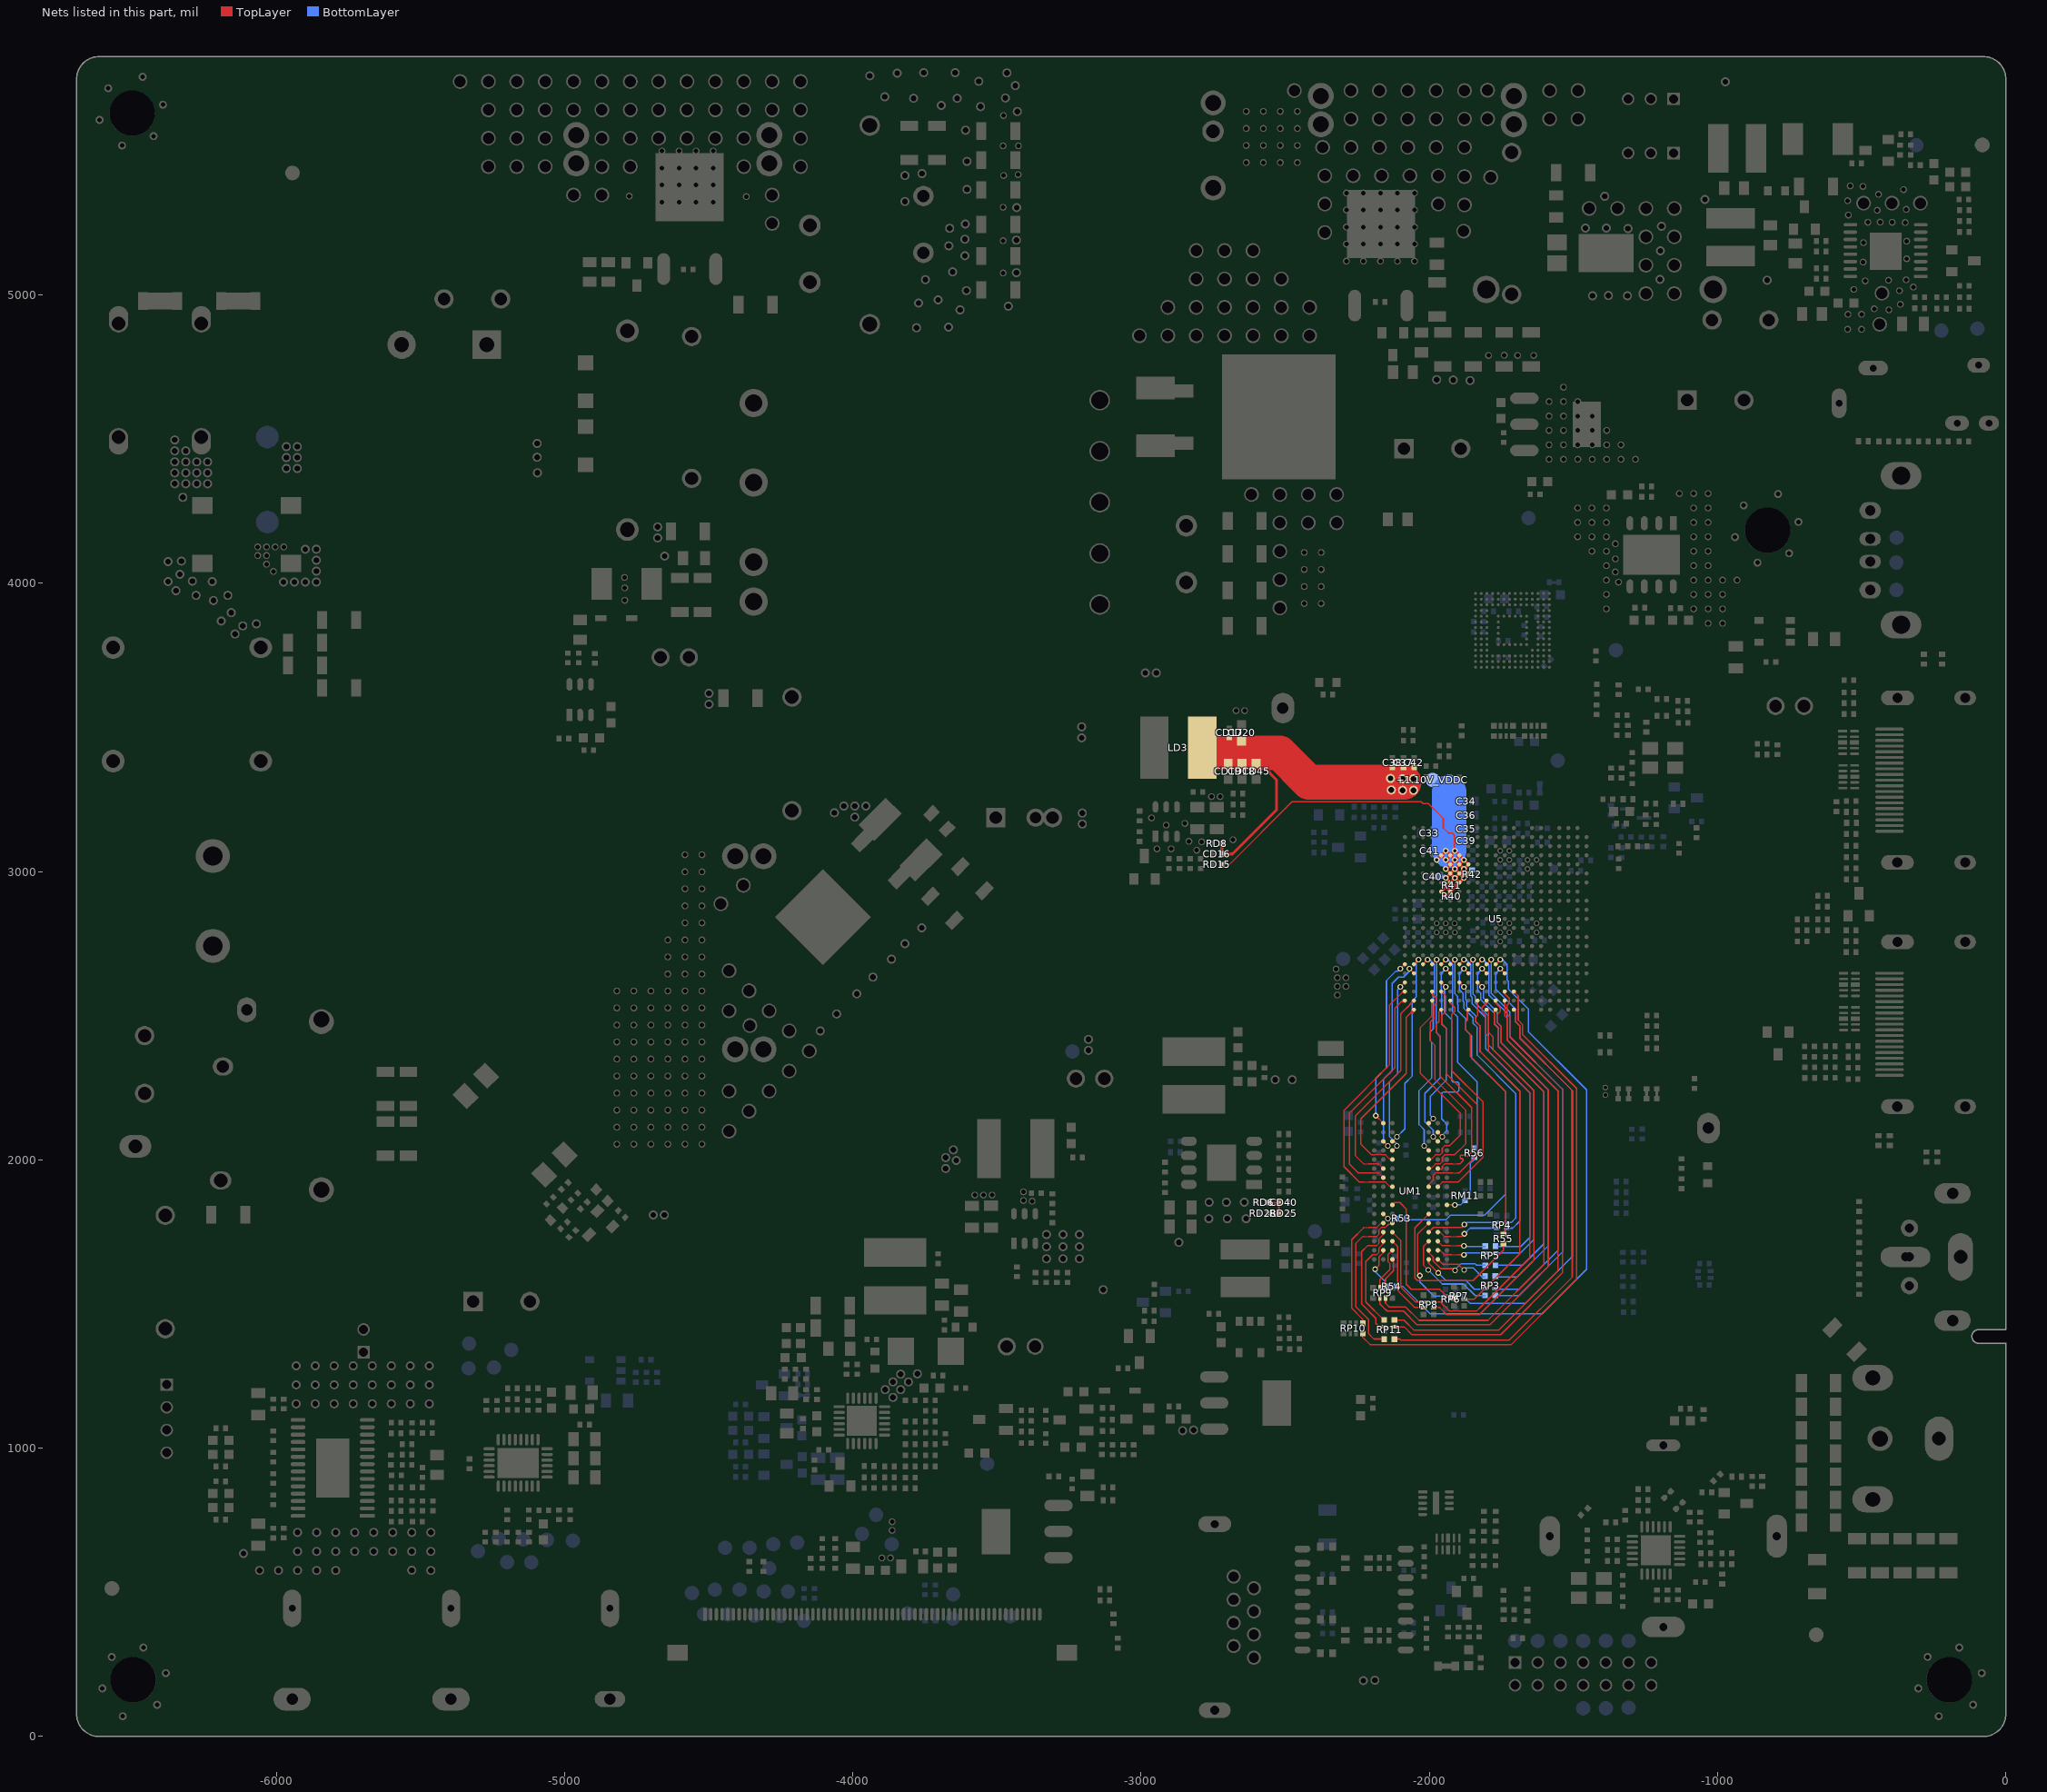
[diagram p0: the nets of this part, all layers, seen from the top]
# Altium PCB MISC84395.PcbDoc (part 10 of 26)
Units mil, origin at the board's own origin, x right, y up, seen from the top; angles counter-clockwise.
Board outline 6692.91 x 5826.77 mil, 2 copper layers (TopLayer, BottomLayer), stack 61.855 mil thick; 951 components, 565 nets, 4374 pads, 1804 vias.
Unrouted connection lines stored in the file: 1.

## Via types
v1: diameter 19.68, hole 11.81, TopLayer to BottomLayer, tented both sides, 1262 vias
v2: diameter 23.62, hole 15.75, TopLayer to BottomLayer, tented both sides, 524 vias
v3: diameter 31.5, hole 19.68, TopLayer to BottomLayer, tented both sides, 11 vias
v4: diameter 24, hole 16, TopLayer to BottomLayer, tented both sides, 6 vias
v5: diameter 19, hole 11.81, TopLayer to BottomLayer, tented both sides, 1 vias

## Nets (pads, with @x,y where several pads share a name; then routed paths per layer and width w, separated by ;. In a path a pad name is that pad's centre, name@x,y a point inside that pad or via, vN(x,y) a via of type N, cw(c..) or ccw(c..) an arc to the next point about the centre after c; other vN are vias at no path point) (continued)
+1.10V_VDDC: +1.10V_VDDC.1 C33.2 C34.2 C35.2 C36.2 C37.2 C38.2 C39.2 C40.2 C41.2 C42.2 CD16.2 CD17.1 CD18.1 CD19.1 CD20.1 CD45.1 LD3.2 pad.VIA5@-1880.2,2977.82 pad.VIA5@-1880.2,3009.31 pad.VIA5@-1880.2,3040.81 pad.VIA5@-1911.7,2977.82 pad.VIA5@-1911.7,3009.31 pad.VIA5@-1911.7,3040.81 pad.VIA5@-1911.7,3072.3 pad.VIA5@-1943.2,2977.82 pad.VIA5@-1943.2,3009.31 pad.VIA5@-1943.2,3040.81 pad.VIA5@-1943.2,3072.3 pad.VIA5@-1974.69,3040.81 pad.VIA5@-2055,3282 pad.VIA5@-2055,3322 pad.VIA5@-2093,3282 pad.VIA5@-2093,3322 pad.VIA5@-2132,3283 pad.VIA5@-2135,3323 R40.1 R41.1 R42.1 RD8.2 RD15.1 U5.P16 U5.P17 U5.R15 U5.R16 U5.T14 U5.T15 U5.T16 U5.U14 U5.U15 U5.U16 U5.V15 U5.V16 U5.V17 | length 3367.3
  TopLayer w5: RD15.1@-2720.27,3025.92 RD15.1@-2720.27,3024.19 -2694.01,3024.19 -2476.38,3241.82 -2028.06,3241.82 -2021.58,3235.34 -2002.82,3235.34 -1951.87,3184.4 -1951.87,3151.49 -1934.52,3134.14 -1921.41,3134.14 -1912.86,3125.59 -1912.86,3073.47 pad.VIA5@-1911.7,3072.3
  TopLayer w10: RD8.2@-2720.18,3097.93 CD16.2@-2720.18,3060.93 -2683.07,3060.93 -2530,3214 -2530,3318 -2575,3363 ; pad.VIA5@-1973.76,3041.74 U5.V17@-1958.94,3056.56 ; -1940.1,2943.22 U5.P16@-1927.45,2930.57 ; -1914.8,2949.42 U5.R16@-1927.45,2962.07 ; U5.V17@-1958.94,3056.56 pad.VIA5@-1943.2,3040.81 ; U5.V17@-1958.94,3056.56 pad.VIA5@-1943.2,3072.3 U5.V16@-1927.45,3056.56 ; pad.VIA5@-1943.2,3040.81 U5.V16@-1927.45,3056.56 ; pad.VIA5@-1943.2,3040.81 U5.U16@-1927.45,3025.06 ; U5.P16@-1927.45,2930.57 -1940.1,2917.92 -1946.3,2917.92 U5.P17@-1958.94,2930.57 U5.R16@-1927.45,2962.07 ; U5.P16@-1927.45,2930.57 -1908.6,2949.42 U5.R15@-1895.95,2962.07 ; U5.R16@-1927.45,2962.07 pad.VIA5@-1911.7,2977.82 ; U5.R16@-1927.45,2962.07 pad.VIA5@-1943.2,2977.82 U5.T16@-1927.45,2993.56 ; U5.T16@-1927.45,2993.56 pad.VIA5@-1911.7,3009.31 ; U5.T16@-1927.45,2993.56 pad.VIA5@-1911.7,2977.82 ; U5.T16@-1927.45,2993.56 pad.VIA5@-1943.2,3009.31 U5.U16@-1927.45,3025.06 ; U5.U16@-1927.45,3025.06 pad.VIA5@-1911.7,3040.81 ; U5.U16@-1927.45,3025.06 pad.VIA5@-1911.7,3009.31 ; U5.V16@-1927.45,3056.56 pad.VIA5@-1911.7,3040.81 ; U5.V16@-1927.45,3056.56 pad.VIA5@-1911.7,3072.3 U5.V15@-1895.95,3056.56 ; pad.VIA5@-1911.7,2977.82 U5.T15@-1895.95,2993.56 ; pad.VIA5@-1911.7,2977.82 U5.R15@-1895.95,2962.07 ; pad.VIA5@-1911.7,3009.31 U5.U15@-1895.95,3025.06 ; pad.VIA5@-1911.7,3009.31 U5.T15@-1895.95,2993.56 ; pad.VIA5@-1911.7,3040.81 U5.U15@-1895.95,3025.06 ; pad.VIA5@-1911.7,3040.81 U5.V15@-1895.95,3056.56 ; U5.R15@-1895.95,2962.07 pad.VIA5@-1880.2,2977.82 ; U5.T15@-1895.95,2993.56 pad.VIA5@-1880.2,2977.82 ; U5.T15@-1895.95,2993.56 pad.VIA5@-1880.2,3009.31 ; U5.U15@-1895.95,3025.06 pad.VIA5@-1880.2,3040.81 ; U5.U15@-1895.95,3025.06 pad.VIA5@-1880.2,3009.31 ; U5.V15@-1895.95,3056.56 pad.VIA5@-1880.2,3040.81 ; pad.VIA5@-1880.2,2977.82 U5.T14@-1864.46,2993.56 pad.VIA5@-1880.2,3009.31 ; pad.VIA5@-1880.2,3009.31 U5.U14@-1864.46,3025.06 pad.VIA5@-1880.2,3040.81
  TopLayer w120: LD3.2@-2774,3411.19 -2519.19,3411.19 -2418,3310 pad.VIA5@-2087,3310
  BottomLayer w12: -1931.35,3072.32 -1925.03,3066
  BottomLayer w15: C40.2@-1972.27,2982 pad.VIA5@-1947.38,2982
  BottomLayer w120: -1931.35,3072.32 -1931.35,3144.15 ; -1931.35,3146.15 -1931.35,3244.15 ; -1931.35,3242.15 -1931.35,3244.15 ; -1931.35,3275.47 -1931.35,3244.15
A2_EN: CD40.1 RD6.1 RD25.1 RD28.1 | length 160.9
  TopLayer w6: RD28.1@-2559.27,1814 RD25.1@-2521.73,1814 ; RD6.1@-2559.27,1851.73 RD6.1@-2559,1852 -2514.84,1852 -2521.73,1845.11 RD25.1@-2521.73,1814 ; CD40.1@-2521.73,1852 RD25.1@-2521.73,1814
A_DDR3_A0: RP8.3 UM1.N3 | length 302.9
  TopLayer w4.92: UM1.N3@-2128.24,1749.47 -2099.69,1720.92 -2099.69,1559.01 -2048.02,1507.34 RP8.3@-2020.46,1507.34
A_DDR3_A0_IC: RP8.4 U5.B12 | length 1382
  TopLayer w3.94: -1816.72,2513.74 -1817.21,2514.23 -1817.21,2528.99 -1801.47,2544.74 U5.B12@-1801.46,2552.62
  TopLayer w4.92: RP8.4@-1977.15,1507.34 -1961.9,1507.34 -1932.37,1477.82 -1930.81,1476.26 -1835.5,1476.26 -1821.52,1490.24 -1651.86,1659.9 -1651.86,2233.23 -1794.58,2375.94 -1794.58,2427.62 -1804.42,2437.46 -1804.42,2501.43 -1816.72,2513.74
A_DDR3_A1: RP3.1 UM1.P7 | length 349
  TopLayer w4.92: v1(-2003.73,1618.07) -2020.95,1635.29 -2020.95,1699.27 UM1.P7@-2002.25,1717.97
  BottomLayer w4.92: v1(-2003.73,1618.07) -1955.15,1569.49 -1881.34,1569.49 -1840.84,1529 RP3.1@-1806.38,1529
A_DDR3_A1_IC: RP3.2 U5.F12 | length 1426.2
  TopLayer w4.92: U5.F12@-1801.46,2678.6 v1(-1785.72,2694.35)
  BottomLayer w3.94: v1(-1785.72,2694.35) -1785.72,2578.7 -1785.23,2578.21
  BottomLayer w4.92: -1785.23,2578.21 -1720.76,2513.74 -1720.76,2427.62 -1538.67,2245.53 -1538.67,1679.59 -1689.26,1529 RP3.2@-1763.08,1529
A_DDR3_A2: RP8.5 UM1.P3 | length 292.5
  TopLayer w4.92: UM1.P3@-2128.24,1717.97 -2109.54,1699.27 -2109.54,1546.72 -2050.48,1487.66 RP8.5@-2020.46,1487.66
A_DDR3_A2_IC: RP8.6 U5.A12 | length 1365.4
  TopLayer w4.92: RP8.6@-1977.15,1487.66 -1964.36,1487.66 -1939.75,1463.05 -1826.55,1463.05 -1637.1,1652.52 -1637.1,2240.61 -1779.81,2383.32 -1779.81,2427.62 -1794.58,2442.38 -1794.58,2514.23 U5.A12@-1801.46,2521.12
A_DDR3_A3: RP11.3 UM1.N2 | length 418.6
  TopLayer w4.92: UM1.N2@-2159.73,1749.47 -2159.73,1741.59 -2175.48,1725.84 -2175.48,1710.1 -2183.36,1702.22 -2214.85,1702.22 -2235.03,1682.04 -2235.03,1499.96 -2185.81,1450.75 -2185.81,1433.52 -2173.51,1421.22 RP11.3@-2158.25,1421.22
A_DDR3_A3_IC: RP11.4 U5.C10 | length 1741.3
  TopLayer w3.94: U5.C10@-1738.47,2584.12 -1738.47,2576.24 -1722.73,2560.49 -1722.73,2544.74 -1730.6,2536.87 -1730.6,2506.36 -1730.11,2505.86
  TopLayer w4.92: RP11.4@-2114.95,1421.22 -2087.39,1421.22 -2060.32,1394.15 -1752.74,1394.15 -1538.67,1608.23 -1538.67,2245.53 -1720.76,2427.62 -1720.76,2496.51 -1730.11,2505.86
A_DDR3_A4: RP5.7 UM1.P8 | length 171.9
  TopLayer w3.94: -1927.45,1702.22 -1903.83,1702.23
  TopLayer w4.92: UM1.P8@-1970.75,1717.97 -1955.01,1702.22 -1927.45,1702.22 ; -1903.83,1702.23 v1(-1880.2,1702.23)
  BottomLayer w4.92: v1(-1880.2,1702.23) -1877.74,1699.77 RP5.7@-1806.38,1699.77
A_DDR3_A4_IC: RP5.8 U5.F15 | length 1208.8
  TopLayer w4.92: U5.F15@-1895.95,2678.6 v1(-1880.21,2694.35)
  BottomLayer w3.94: v1(-1880.21,2694.35) -1872.33,2694.35 -1856.58,2678.6 -1856.58,2568.36 -1856.09,2567.87
  BottomLayer w4.92: -1856.09,2567.87 -1851.17,2562.95 -1851.17,2540.8 -1804.42,2494.05 -1804.42,2385.78 -1651.86,2233.23 -1651.86,1731.26 -1683.35,1699.77 RP5.8@-1763.08,1699.77
A_DDR3_A5: RP11.1 UM1.P2 | length 332.9
  TopLayer w4.92: UM1.P2@-2159.73,1717.97 -2159.73,1710.1 -2175.48,1694.35 -2175.48,1678.6 -2183.36,1670.73 -2197.14,1670.73 -2220.26,1647.61 -2220.26,1507.34 -2158.25,1445.34 RP11.1@-2158.25,1443.86
A_DDR3_A5_IC: RP11.2 U5.B10 | length 1675.3
  TopLayer w3.94: U5.B10@-1738.47,2552.62 -1738.47,2499.47 -1737.98,2498.97
  TopLayer w4.92: RP11.2@-2114.95,1443.86 -2087.88,1443.86 -2052.94,1408.92 -1760.12,1408.92 -1553.43,1615.62 -1553.43,2238.15 -1730.6,2415.31 -1730.6,2491.59 -1737.98,2498.97
A_DDR3_A6: RP5.5 UM1.R8 | length 173.5
  TopLayer w3.94: -1923.51,1670.73 -1899.89,1670.73
  TopLayer w4.92: UM1.R8@-1970.75,1686.48 -1962.88,1686.47 -1947.14,1670.73 -1923.51,1670.73 ; -1899.89,1670.73 v1(-1880.2,1670.73)
  BottomLayer w4.92: v1(-1880.2,1670.73) -1873.81,1677.13 RP5.5@-1806.38,1677.13
A_DDR3_A6_IC: RP5.6 U5.F14 | length 1225.7
  TopLayer w4.92: U5.F14@-1864.46,2678.6 v1(-1848.71,2694.35)
  BottomLayer w3.94: v1(-1848.71,2694.35) -1848.71,2575.25 -1848.22,2574.76
  BottomLayer w4.92: -1848.22,2574.76 -1841.33,2567.87 -1841.33,2545.73 -1794.58,2498.97 -1794.58,2398.09 -1637.1,2240.61 -1637.1,1723.88 -1683.85,1677.13 RP5.6@-1763.08,1677.13
A_DDR3_A7: R54.1 UM1.R2 | length 151
  TopLayer w4.92: v1(-2188.27,1620.53) -2175.48,1633.33 -2175.48,1662.85 -2159.73,1678.6 UM1.R2@-2159.73,1686.48
  BottomLayer w4.92: v1(-2188.27,1620.53) -2188.27,1613.15 -2154.14,1579.02 R54.1@-2154.14,1561.48
A_DDR3_A7_IC: R54.2 U5.F11 | length 1987
  TopLayer w4.92: U5.F11@-1769.97,2678.6 v1(-1754.22,2694.35)
  BottomLayer w3.94: v1(-1754.22,2694.35) -1746.35,2694.35 -1730.6,2678.6 -1730.6,2624.47 -1730.11,2623.97
  BottomLayer w4.92: R54.2@-2114.14,1561.48 -2092.31,1561.48 -1998.81,1467.97 -1997.25,1466.42 -1609.12,1466.42 -1590.31,1485.23 -1455.01,1620.53 -1455.01,2243.07 -1656.78,2444.84 -1656.78,2523.58 -1725.68,2592.48 -1725.68,2619.54 -1730.11,2623.97
A_DDR3_A8: RP3.7 UM1.T8 | length 195.8
  TopLayer w4.92: UM1.T8@-1970.75,1654.98 -1953.53,1637.75 -1900.38,1637.75 v1@-1880.7,1618.07
  BottomLayer w4.92: v1@-1880.7,1618.07 -1873.31,1625.45 -1848.22,1625.45 -1816.72,1593.96 RP3.7@-1806.38,1593.96
  other v1: -1879.24,1618.32
A_DDR3_A8_IC: RP3.8 U5.D13 | length 1235.2
  TopLayer w4.92: U5.D13@-1832.96,2615.61 v1(-1817.21,2599.86)
  BottomLayer w4.92: v1(-1817.21,2599.86) -1811.8,2594.45 -1811.8,2560.49 -1765.05,2513.74 -1765.05,2476.83 -1750.28,2462.06 -1750.28,2405.47 -1587.88,2243.07 -1587.88,1701.74 -1695.66,1593.96 RP3.8@-1763.08,1593.96
A_DDR3_A9: RP9.5 UM1.R3 | length 154.5
  TopLayer w4.92: RP9.5@-2171.67,1556.06 -2171.67,1585.46 -2159.17,1597.97 -2136.6,1620.53 -2136.6,1640.22 -2143.99,1647.6 -2143.99,1670.73 UM1.R3@-2128.24,1686.48
A_DDR3_A9_IC: RP9.6 U5.B11 | length 1723.9
  TopLayer w3.94: U5.B11@-1769.97,2552.62 -1769.97,2544.74 -1754.22,2528.99 -1754.22,2514.72 -1754.71,2514.23
  TopLayer w4.92: RP9.6@-2171.67,1520.63 -2171.67,1500.58 -2162.86,1491.77 -2146.44,1475.36 -2089.85,1475.36 -2043.1,1428.6 -1789.65,1428.6 -1587.88,1630.38 -1587.88,2243.07 -1750.28,2405.47 -1750.28,2462.06 -1765.05,2476.83 -1765.05,2503.89 -1754.71,2514.23
A_DDR3_A10: R55.1 UM1.L7 | length 618.7
  TopLayer w4.92: UM1.L7@-2002.25,1812.46 -2050.48,1764.23 -2050.48,1591 -2040.64,1581.16 -1848.71,1581.16 -1742.9,1686.97 R55.1@-1742.9,1708.8
A_DDR3_A10_IC: R55.2 U5.A14 | length 836.1
  TopLayer w4.92: U5.A14@-1864.46,2521.12 -1868.4,2517.18 -1868.4,2484.21 -1873.32,2479.29 -1873.32,2449.76 -1858.55,2435 -1858.55,2358.72 -1735.52,2235.69 -1735.52,1756.18 R55.2@-1742.9,1748.8
A_DDR3_A11: RP5.1 UM1.R7 | length 248.3
  TopLayer w4.92: UM1.R7@-2002.25,1686.48 -2002.25,1678.6 -1986.51,1662.85 -1986.51,1649.07 -1960.42,1622.99 -1917.61,1622.99 v1@-1912.69,1618.07
  BottomLayer w4.92: v1@-1912.69,1618.07 -1890.54,1640.21 -1841.81,1640.21 -1836.4,1634.8 RP5.1@-1806.38,1634.8
  other v1: -1910.63,1617.05
A_DDR3_A11_IC: RP5.2 U5.E12 | length 1269.1
  TopLayer w4.92: v1(-1817.21,2662.85) U5.E12@-1801.46,2647.11
  BottomLayer w3.94: -1832.47,2588.54 -1832.96,2589.03 -1832.96,2647.1 v1(-1817.21,2662.85)
  BottomLayer w4.92: -1832.47,2588.54 -1821.64,2577.71 -1821.64,2555.57 -1774.89,2508.82 -1774.89,2471.91 -1760.13,2457.14 -1760.13,2393.17 -1602.65,2235.69 -1602.65,1709.11 -1676.96,1634.8 RP5.2@-1763.08,1634.8
A_DDR3_A12: RP4.5 UM1.N7 | length 244.2
  TopLayer w4.92: UM1.N7@-2002.25,1749.47 -1986.01,1765.71 -1888.07,1765.71 v1(-1878.24,1775.55)
  BottomLayer w4.92: v1(-1878.24,1775.55) -1870.85,1782.93 RP4.5@-1771.94,1782.93
A_DDR3_A12_IC: RP4.6 U5.E14 | length 1008.3
  TopLayer w4.92: v1(-1880.21,2662.85) U5.E14@-1864.46,2647.11
  BottomLayer w3.94: -1895.46,2590.02 -1895.95,2590.51 -1895.95,2647.1 v1(-1880.21,2662.85)
  BottomLayer w4.92: -1895.46,2590.02 -1883.16,2577.71 -1883.16,2550.65 -1880.7,2548.19 -1880.7,2526.04 -1848.71,2494.05 -1848.71,2474.37 -1833.95,2459.6 -1833.95,2363.64 -1701.07,2230.77 -1701.07,1797.7 -1715.83,1782.93 RP4.6@-1728.63,1782.93
A_DDR3_A13: RP9.3 UM1.T3 | length 112
  TopLayer w4.92: RP9.3@-2151.98,1556.06 -2151.98,1587.93 -2141.12,1598.79 -2124.3,1615.61 -2124.3,1651.04 UM1.T3@-2128.24,1654.98
A_DDR3_A13_IC: RP9.4 U5.A11 | length 1628.9
  TopLayer w4.92: RP9.4@-2151.98,1520.63 -2151.98,1503.04 -2139.06,1490.12 -2082.47,1490.12 -2035.72,1443.37 -1797.03,1443.37 -1602.65,1637.75 -1602.65,2235.69 -1760.13,2393.17 -1760.13,2457.14 -1774.89,2471.91 -1774.89,2516.2 U5.A11@-1769.97,2521.12
A_DDR3_A14: RP3.3 UM1.T7 | length 246.7
  TopLayer w4.92: UM1.T7@-2002.25,1654.98 -2002.25,1641.2 v1(-1969.28,1608.23)
  BottomLayer w4.92: v1(-1969.28,1608.23) -1942.21,1581.16 -1873.31,1581.16 -1843.79,1551.64 RP3.3@-1806.38,1551.64
A_DDR3_A14_IC: RP3.4 U5.F13 | length 1407.5
  TopLayer w4.92: U5.F13@-1832.96,2678.6 v1(-1817.21,2694.35)
  BottomLayer w3.94: v1(-1817.21,2694.35) -1812.24,2694.35 -1793.59,2675.7 -1793.59,2571.81 -1793.1,2571.32
  BottomLayer w4.92: -1793.1,2571.32 -1730.6,2508.82 -1730.6,2415.31 -1553.43,2238.15 -1553.43,1686.97 -1688.77,1551.64 RP3.4@-1763.08,1551.64
A_DDR3_A15: RP6.5 UM1.M7 | length 325.8
  TopLayer w4.92: v1(-2033.26,1598.39) -2040.64,1605.77 -2040.64,1742.58 UM1.M7@-2002.25,1780.97
  BottomLayer w4.92: v1(-2033.26,1598.39) -2033.26,1576.24 -1984.04,1527.03 RP6.5@-1951.56,1527.03
A_DDR3_A15_IC: RP6.6 U5.E10 | length 1632.2
  TopLayer w4.92: v1(-1754.22,2662.85) U5.E10@-1738.47,2647.11
  BottomLayer w3.94: -1769.48,2591.99 -1769.97,2592.48 -1769.97,2647.1 v1(-1754.22,2662.85)
  BottomLayer w4.92: RP6.6@-1908.26,1527.03 -1883.16,1527.03 -1858.55,1502.42 -1680.47,1502.42 ; -1769.48,2591.99 -1701.46,2523.98 -1701.46,2479.69 -1686.31,2464.52 -1686.31,2422.69 -1504.22,2240.61 -1504.22,1664.83 -1666.63,1502.42 ; -1680.47,1502.42 -1666.63,1502.42 ; -1680.47,1502.42 -1666.63,1502.42
A_DDR3_BA0: RP10.1 UM1.M2 | length 439.4
  TopLayer w3.94: -2226.66,1765.21 -2210.91,1765.21
  TopLayer w4.92: RP10.1@-2232.07,1433.03 -2232.07,1448.29 -2269.48,1485.69 -2269.48,1723.39 -2227.65,1765.21 -2226.66,1765.21 ; -2210.91,1765.21 -2183.36,1765.21 -2167.61,1780.96 UM1.M2@-2159.73,1780.97
A_DDR3_BA0_IC: RP10.2 U5.C9 | length 1939
  TopLayer w4.92: RP10.2@-2232.07,1389.73 -2232.07,1386.28 -2205.5,1359.71 -1715.83,1359.71 -1489.46,1586.08 -1489.46,2247.99 -1676.47,2435 -1676.47,2469.45 -1691.82,2484.8 -1691.82,2568.95 U5.C9@-1706.98,2584.12
A_DDR3_BA1: RP4.3 UM1.N8 | length 217.6
  TopLayer w3.94: -1927.45,1733.72 -1903.83,1733.72
  TopLayer w4.92: UM1.N8@-1970.75,1749.47 -1962.88,1749.47 -1947.14,1733.72 -1927.45,1733.72 ; -1903.83,1733.72 -1888.08,1733.72 v1(-1878.24,1743.56)
  BottomLayer w4.92: v1(-1878.24,1743.56) -1858.55,1763.25 RP4.3@-1771.94,1763.25
A_DDR3_BA1_IC: RP4.4 U5.D15 | length 967.1
  TopLayer w4.92: U5.D15@-1895.95,2615.61 v1(-1880.21,2599.86)
  BottomLayer w4.92: v1(-1880.21,2599.86) -1873.32,2592.97 -1873.32,2555.57 -1870.86,2553.11 -1870.86,2530.96 -1838.87,2498.97 -1838.87,2479.29 -1824.1,2464.52 -1824.1,2375.94 -1686.31,2238.15 -1686.31,1787.85 -1710.91,1763.25 RP4.4@-1728.63,1763.25
A_DDR3_BA2: RP11.7 UM1.M3 | length 557
  TopLayer w3.94: -2226.66,1733.72 -2210.91,1733.72
  TopLayer w4.92: -2226.66,1733.72 -2232.08,1733.72 -2254.71,1711.09 -2254.71,1490.12 -2210.42,1445.83 -2210.42,1396.62 -2192.7,1378.9 RP11.7@-2158.25,1378.9 ; -2210.91,1733.72 -2183.36,1733.72 -2175.48,1741.59 -2175.48,1757.34 -2167.61,1765.21 -2153.83,1765.21 -2142.02,1777.02 -2132.17,1777.02 UM1.M3@-2128.24,1780.97
A_DDR3_BA2_IC: RP11.8 U5.A9 | length 1714.9
  TopLayer w4.92: RP11.8@-2114.95,1378.9 -2101.66,1378.9 -2097.23,1374.47 -1723.22,1374.47 -1504.22,1593.47 -1504.22,2240.61 -1686.31,2422.69 -1686.31,2464.52 -1701.46,2479.69 -1701.46,2515.61 U5.A9@-1706.98,2521.12
A_DDR3_CASZ: RP7.5 UM1.K3 | length 508.6
  TopLayer w4.92: UM1.K3@-2128.24,1843.96 -2119.87,1852.32 -2102.65,1852.32 -2080.01,1829.68 -2080.01,1568.86 -2079.97,1568.82 ; -2079.93,1568.86 -2062.62,1551.56 -1964.28,1551.56 -1929.91,1517.19 RP7.5@-1914.65,1517.19
A_DDR3_CASZ_IC: RP7.6 U5.B13 | length 1193.9
  TopLayer w3.94: -1833.45,2499.47 -1832.96,2499.96 U5.B13@-1832.96,2552.62
  TopLayer w4.92: RP7.6@-1871.35,1517.19 -1843.79,1517.19 -1686.31,1674.67 -1686.31,2238.15 -1824.1,2375.94 -1824.1,2464.52 -1838.87,2479.29 -1838.87,2494.05 -1833.45,2499.47
A_DDR3_CKE: R56.1 RM11.2 UM1.K9 | length 225.1
  TopLayer w4.92: UM1.K9@-1939.26,1843.96 v1(-1911.7,1843.95)
  BottomLayer w4.92: v1(-1911.7,1843.95) -1891.7,1843.95 -1880.2,1855.45 -1876.27,1859.39 -1858.55,1877.11 -1858.55,1986.85 R56.1@-1843.79,2001.62
A_DDR3_CKE_IC: R56.2 U5.F17 | length 729.4
  TopLayer w4.92: U5.F17@-1958.94,2678.6 v1(-1943.2,2694.35)
  BottomLayer w3.94: v1(-1943.2,2694.35) -1935.32,2694.35 -1919.58,2678.6 -1919.58,2583.13 -1920.07,2582.64
  BottomLayer w4.92: -1920.07,2582.64 -1920.07,2513.74 -1902.84,2496.51 -1902.84,2339.03 -1833.95,2270.14 -1833.95,2051.45 R56.2@-1843.79,2041.62
A_DDR3_CSB0: R53.1 UM1.L2 | length 53.5
  TopLayer w4.92: UM1.L2@-2159.73,1812.46 v1(-2143.99,1796.71)
  BottomLayer w4.92: v1(-2143.99,1796.71) R53.1@-2112.8,1796.71
A_DDR3_CSB0_IC: R53.2 U5.F16 | length 1283.8
  TopLayer w4.92: U5.F16@-1927.45,2678.6 v1(-1911.7,2694.35)
  BottomLayer w3.94: v1(-1911.7,2694.35) -1911.7,2576.73 -1911.21,2576.24
  BottomLayer w4.92: R53.2@-2072.8,1796.71 -2068.86,1792.78 -1942.21,1792.78 -1927.45,1807.54 -1809.34,1807.54 -1735.52,1881.36 -1735.52,2235.69 -1853.63,2353.8 -1853.63,2430.08 -1873.32,2449.76 -1873.32,2489.13 -1900.38,2516.2 -1900.38,2538.34 -1902.84,2540.8 -1902.84,2567.87 -1911.21,2576.24
A_DDR3_DM0_IC: U5.B18 UM1.E7 | length 693.9
  TopLayer w3.94: -1992.9,2497.5 -1992.41,2497.99 -1992.41,2550.65 U5.B18@-1990.44,2552.62
  TopLayer w4.92: UM1.E7@-2002.25,2001.44 -1994.38,2001.43 -1978.63,2017.18 -1962.88,2017.18 -1955.01,2025.06 -1955.01,2040.8 -1947.14,2048.68 -1930.4,2048.68 -1893,2086.08 -1893,2161.87 -2030.8,2299.66 -2030.8,2459.6 -1992.9,2497.5
A_DDR3_DM1_IC: U5.D21 UM1.D3 | length 622.6
  TopLayer w4.92: UM1.D3@-2128.24,2032.93 v1(-2112.49,2048.68) ; v1(-2100.68,2599.86) U5.D21@-2084.93,2615.61
  BottomLayer w4.92: v1(-2112.49,2048.68) -2112.49,2055.65 -2139.06,2082.22 -2139.06,2270.14 -2109.54,2299.66 -2109.54,2591 v1(-2100.68,2599.86)
A_DDR3_DQ0_IC: U5.A20 UM1.E3 | length 674.7
  TopLayer w4.92: UM1.E3@-2128.24,2001.44 -2136.11,2001.43 -2151.86,2017.18 -2200.09,2017.18 -2237.49,2054.58 -2237.49,2142.18 -2080.01,2299.66 -2080.01,2494.54 -2059.67,2514.88
  TopLayer w12: -2058.52,2513.73 -2053.43,2518.81 U5.A20@-2053.43,2521.12
A_DDR3_DQ1_IC: U5.C18 UM1.F7 | length 768.1
  TopLayer w3.94: U5.C18@-1990.44,2584.12 -1990.44,2576.24 -1974.69,2560.49 -1974.69,2544.74 -1984.54,2534.9 -1984.54,2491.1 -1985.03,2490.61
  TopLayer w4.92: UM1.F7@-2002.25,1969.94 -1994.38,1969.94 -1978.63,1985.69 -1962.88,1985.69 -1955.01,1993.56 -1955.01,2009.31 -1946.64,2017.67 -1912.19,2017.67 -1873.32,2056.55 -1873.32,2171.71 -1981.58,2279.98 -1981.58,2398.09 -1996.35,2412.85 -1996.35,2479.29 -1985.03,2490.61
A_DDR3_DQ2_IC: U5.B20 UM1.F2 | length 738
  TopLayer w3.94: -2226.66,1985.69 -2210.91,1985.69 ; -2080.99,2525.06 U5.B20@-2056.21,2549.84
  TopLayer w4.92: -2226.66,1985.69 -2227.65,1985.69 -2257.17,2015.21 -2257.17,2152.02 -2099.69,2309.51 -2099.69,2506.36 -2080.99,2525.06 ; -2210.91,1985.69 -2175.48,1985.69 UM1.F2@-2159.73,1969.94
  TopLayer w12: U5.B20@-2056.21,2549.84 U5.B20@-2053.43,2552.62
A_DDR3_DQ3_IC: U5.A17 UM1.F8 | length 730
  TopLayer w3.94: -1919.58,1985.69 -1903.83,1985.69
  TopLayer w4.92: UM1.F8@-1970.75,1969.94 -1968.3,1967.48 -1959.93,1967.48 ccw(c-1959.93,1972.4) -1955.01,1972.4 -1955.01,1977.82 -1947.14,1985.69 -1919.58,1985.69 ; U5.A17@-1958.94,2521.12 -1966.82,2513.25 -1966.82,2479.29 -1976.66,2469.45 -1976.66,2442.38 -1961.9,2427.62 -1961.9,2289.82 -1853.63,2181.55 -1853.63,2026.54 -1867.91,2012.26 -1871.34,2012.26 -1875.77,2016.69 -1890.54,2016.69 -1893,2014.23 -1893,2006.85 -1890.54,2004.39 -1885.62,2004.39 -1883.16,2001.93 -1883.16,1997.01 -1894.47,1985.69 -1903.83,1985.69
A_DDR3_DQ4_IC: U5.C21 UM1.H3 | length 894.5
  TopLayer w3.94: -2226.66,1922.69 -2210.91,1922.69
  TopLayer w4.92: -2226.66,1922.69 -2242.41,1922.69 -2296.54,1976.83 -2296.54,2171.71 -2139.06,2329.19 -2139.06,2535.88 U5.C21@-2090.84,2584.11 ; -2210.91,1922.69 -2151.86,1922.69 -2136.11,1906.95 UM1.H3@-2128.24,1906.95
  TopLayer w12: U5.C21@-2088.89,2582.17 -2086.95,2584.11 U5.C21@-2084.93,2584.12
A_DDR3_DQ5_IC: U5.B16 UM1.H8 | length 798.1
  TopLayer w3.94: U5.B16@-1927.45,2552.62 -1927.45,2544.74 -1911.7,2528.99 -1911.7,2514.72 -1912.19,2514.23 ; -1919.58,1922.69 -1903.83,1922.69
  TopLayer w4.92: UM1.H8@-1970.75,1906.95 -1955.01,1922.69 -1919.58,1922.69 ; -1912.19,2514.23 -1922.53,2503.89 -1922.53,2309.51 -1814.26,2201.24 -1814.26,2009.31 -1900.88,1922.69 -1903.83,1922.69
A_DDR3_DQ6_IC: U5.B21 UM1.G2 | length 788.6
  TopLayer w3.94: -2226.66,1954.19 -2210.91,1954.19
  TopLayer w4.92: -2226.66,1954.19 -2245.36,1954.19 -2276.86,1985.69 -2276.86,2161.87 -2119.38,2319.35 -2119.38,2526.04 -2092.8,2552.62 U5.B21@-2090.66,2552.62 ; -2210.91,1954.19 -2175.48,1954.19 UM1.G2@-2159.73,1938.45
  TopLayer w12: U5.B21@-2090.66,2550.49 -2088.53,2552.62 U5.B21@-2084.93,2552.62
A_DDR3_DQ7_IC: U5.C17 UM1.H7 | length 857.5
  TopLayer w3.94: -1919.58,1954.19 -1903.83,1954.19
  TopLayer w4.92: UM1.H7@-2002.25,1906.95 -2002.25,1914.82 -1986.51,1930.57 -1986.51,1946.32 -1978.63,1954.19 -1919.58,1954.19 ; U5.C17@-1958.94,2584.12 -1943.2,2568.36 -1943.2,2515.21 -1956.98,2501.43 -1956.98,2471.91 -1942.21,2457.14 -1942.21,2299.66 -1833.95,2191.39 -1833.95,2017.89 -1897.64,1954.19 -1903.83,1954.19
A_DDR3_DQ8_IC: U5.F19 UM1.D7 | length 738
  TopLayer w4.92: U5.F19@-2021.94,2678.6 v1(-2006.19,2694.35) ; v1(-2018,2048.68) UM1.D7@-2002.25,2032.93
  BottomLayer w3.94: v1(-2006.19,2694.35) -1998.32,2694.35 -1982.57,2678.6 -1982.57,2576.73 -1983.06,2576.24
  BottomLayer w4.92: v1(-2018,2048.68) -2018,2104.78 -2035.72,2122.5 -2035.72,2240.61 -1991.43,2284.9 -1991.43,2407.93 -1996.35,2412.85 -1996.35,2444.84 -1986.51,2454.68 -1986.51,2572.79 -1983.06,2576.24
A_DDR3_DQ9_IC: U5.F20 UM1.C3 | length 689.7
  TopLayer w4.92: UM1.C3@-2128.24,2064.43 v1(-2112.49,2080.17) ; U5.F20@-2053.43,2678.6 v1(-2037.69,2694.35)
  BottomLayer w3.94: -2046.05,2564.92 -2045.56,2565.41 -2045.56,2686.47 v1(-2037.69,2694.35)
  BottomLayer w4.92: v1(-2112.49,2080.17) -2084.93,2107.73 -2084.93,2265.21 -2060.32,2289.82 -2060.32,2550.65 -2046.05,2564.92
A_DDR3_DQ10_IC: U5.F18 UM1.C8 | length 700.3
  TopLayer w4.92: U5.F18@-1990.44,2678.6 v1(-1974.69,2694.35) ; v1(-1986.51,2080.17) UM1.C8@-1970.75,2064.43
  BottomLayer w3.94: -1975.19,2569.35 -1974.69,2569.84 v1(-1974.69,2694.35)
  BottomLayer w4.92: v1(-1986.51,2080.17) -1986.51,2102.81 -2016.03,2132.34 -2016.03,2230.77 -1961.9,2284.9 -1961.9,2427.62 -1976.66,2442.38 -1976.66,2567.87 -1975.19,2569.35
A_DDR3_DQ11_IC: U5.E20 UM1.C2 | length 712
  TopLayer w4.92: UM1.C2@-2159.73,2064.43 v1(-2143.98,2048.68) ; v1(-2069.18,2662.85) U5.E20@-2053.43,2647.11
  BottomLayer w3.94: -2090.84,2634.31 -2089.85,2634.31 -2069.18,2654.98 v1(-2069.18,2662.85)
  BottomLayer w4.92: v1(-2143.98,2048.68) -2158.75,2063.45 -2158.75,2279.98 -2129.22,2309.51 -2129.22,2612.16 -2107.08,2634.31 -2090.84,2634.31
A_DDR3_DQ12_IC: U5.E16 UM1.A7 | length 604.2
  TopLayer w4.92: UM1.A7@-2002.25,2127.42 v1(-1986.51,2143.17) ; v1(-1943.2,2662.85) U5.E16@-1927.45,2647.11
  BottomLayer w3.94: -1958.45,2589.03 -1958.95,2589.52 -1958.95,2647.1 v1(-1943.2,2662.85)
  BottomLayer w4.92: v1(-1986.51,2143.17) -1996.35,2153.01 -1996.35,2220.92 -1942.21,2275.06 -1942.21,2457.14 -1956.98,2471.91 -1956.98,2587.56 -1958.45,2589.03
A_DDR3_DQ13_IC: U5.F21 UM1.A2 | length 608.1
  TopLayer w4.92: v1(-2185.82,2153.5) UM1.A2@-2159.73,2127.42 ; v1(-2100.68,2662.85) U5.F21@-2084.93,2678.6
  BottomLayer w4.92: v1(-2185.82,2153.5) -2185.82,2282.44 -2148.91,2319.35 -2148.91,2622.01 -2116.92,2653.99 -2109.54,2653.99 v1(-2100.68,2662.85)
A_DDR3_DQ14_IC: U5.D17 UM1.B8 | length 663.6
  TopLayer w4.92: UM1.B8@-1970.75,2095.93 v1(-1955.01,2080.18) ; U5.D17@-1958.94,2615.61 v1(-1943.2,2599.86)
  BottomLayer w3.94: -1939.26,2103.8 -1939.26,2119.54
  BottomLayer w4.92: v1(-1955.01,2080.18) -1955.01,2086.08 -1939.26,2101.83 -1939.26,2103.8 ; v1(-1943.2,2599.86) -1947.14,2595.92 -1947.14,2511.28 -1922.53,2486.67 -1922.53,2275.06 -1917.61,2270.14 -1902.06,2270.14 -1897.14,2265.21 -1897.14,2240.61 -1902.06,2235.69 -1952.06,2235.69 -1956.98,2230.77 -1956.98,2142.18 -1939.26,2124.47 -1939.26,2119.54